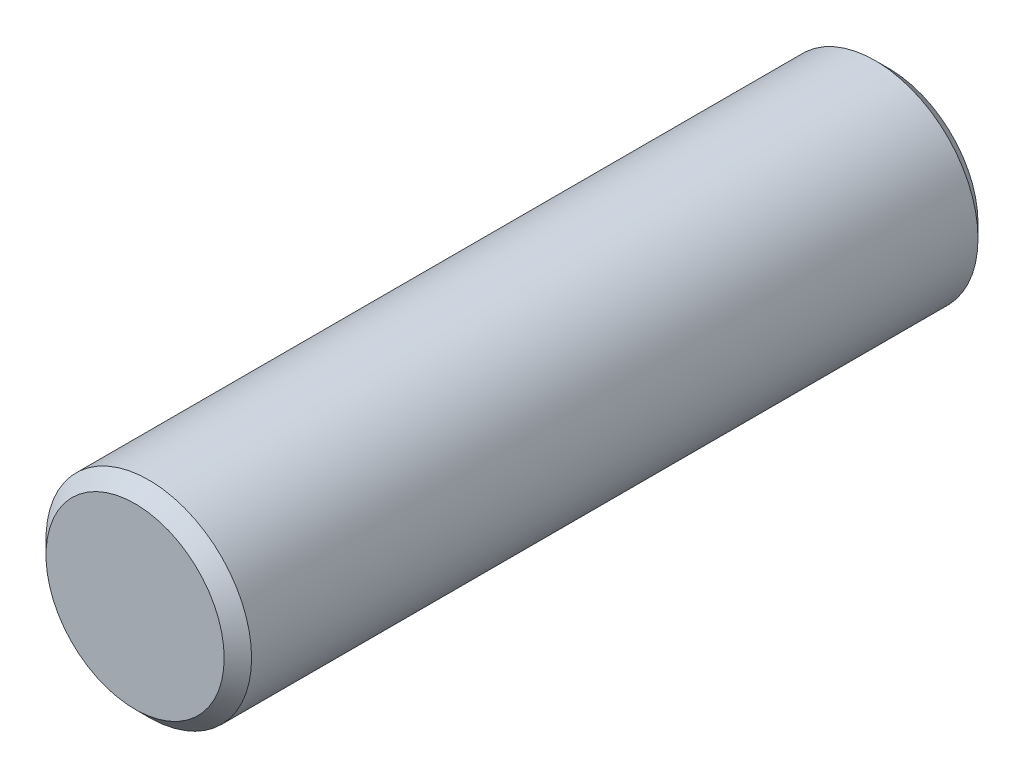
from build123d import *

# Parameters (mm, degrees)
SKETCH1_R           = 1.5
BOSS_EXTRUDE1_DEPTH = 11
CHAMFER1_SIZE       = 0.2


with BuildPart() as part:
    # Sketch1 → Boss-Extrude1 (new body)
    with BuildSketch(Plane.XY):
        with Locations((0, 8.569064594)):
            Circle(SKETCH1_R)
    extrude(amount=-BOSS_EXTRUDE1_DEPTH)

    # Chamfer1
    chamfer1_edges = [part.edges().sort_by_distance(p)[0] for p in [
        (-1.5, 8.569064594, 0),
        (-1.5, 8.569064594, -11),
    ]]
    chamfer(chamfer1_edges, length=CHAMFER1_SIZE)


solid = part.part
